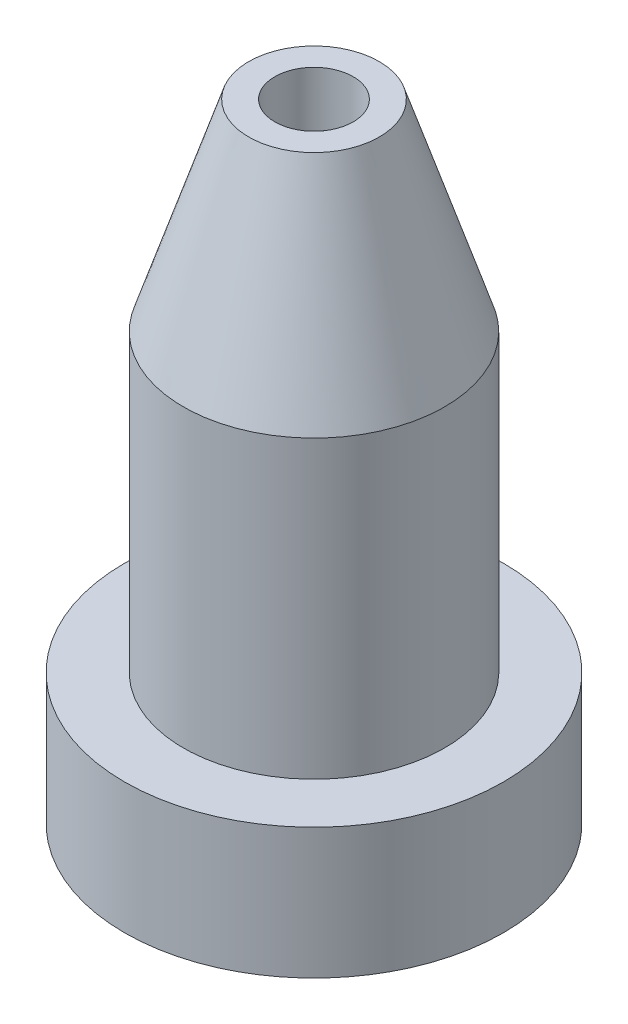
from build123d import *

# Parameters (mm, degrees)
SKETCH1_R           = 1
BOSS_EXTRUDE1_DEPTH = 4.8
SKETCH3_R           = 0.75
CUT_EXTRUDE1_DEPTH  = 3
SKETCH4_R           = 0.3
CUT_EXTRUDE2_DEPTH  = 3
SKETCH5_R           = 0.5
CUT_EXTRUDE3_DEPTH  = 0.6
SKETCH6_R           = 1.45
SKETCH6_R_2         = 1
BOSS_EXTRUDE2_DEPTH = 1
CHAMFER1_SIZE       = 0.3
CHAMFER1_SIZE2      = 1


with BuildPart() as part:
    # Sketch1 → Boss-Extrude1 (new body)
    with BuildSketch(Plane(origin=(0, 0, 0), x_dir=(1, 0, 0), z_dir=(0, 1, 0))):
        with Locations(Location((0, 0, 0), (0, 0, 270))):
            Circle(SKETCH1_R)
    extrude(amount=BOSS_EXTRUDE1_DEPTH)

    # Sketch2 → Cut-Revolve1 (revolve, cut)
    with BuildSketch(Plane.XY, mode=Mode.PRIVATE) as cut_revolve1_sk:
        Polygon((0.5, 4.8), (1.621441373, 1.348558349), (1.621441373, 4.8), align=None)
    revolve(cut_revolve1_sk.sketch.rotate(Axis((0, 0, 0), (0, 1, 0)), 90), axis=Axis((0, 0, 0), (0, 1, 0)), mode=Mode.SUBTRACT)

    # Sketch3 → Cut-Extrude1 (cut)
    with BuildSketch(Plane.XZ):
        with Locations(Location((0, 0, 0), (0, 0, 270))):
            Circle(SKETCH3_R)
    extrude(amount=-CUT_EXTRUDE1_DEPTH, mode=Mode.SUBTRACT)

    # Sketch4 → Cut-Extrude2 (cut)
    with BuildSketch(Plane(origin=(0, 4.8, 0), x_dir=(1, 0, 0), z_dir=(0, 1, 0))):
        with Locations(Location((0, 0, 0), (0, 0, 270))):
            Circle(SKETCH4_R)
    extrude(amount=-CUT_EXTRUDE2_DEPTH, mode=Mode.SUBTRACT)

    # Sketch5 → Cut-Extrude3 (cut)
    with BuildSketch(Plane.XZ.offset(-3)):
        with Locations(Location((0, 0, 0), (0, 0, 270))):
            Circle(SKETCH5_R)
    extrude(amount=-CUT_EXTRUDE3_DEPTH, mode=Mode.SUBTRACT)

    # Sketch6 → Boss-Extrude2 (add)
    with BuildSketch(Plane.XZ):
        with Locations(Location((0, 0, 0), (0, 0, 270))):
            Circle(SKETCH6_R)
        with Locations(Location((0, 0, 0), (0, 0, 270))):
            Circle(SKETCH6_R_2, mode=Mode.SUBTRACT)
    extrude(amount=-BOSS_EXTRUDE2_DEPTH)

    # Chamfer1
    chamfer1_edges = [part.edges().sort_by_distance(p)[0] for p in [
        (0, 0, 0.75),
    ]]
    chamfer1_side = [part.faces().sort_by_distance(p)[0] for p in [
        (0, 0, 1.408987807),
    ]]
    chamfer(chamfer1_edges, length=CHAMFER1_SIZE, length2=CHAMFER1_SIZE2, reference=chamfer1_side[0])


solid = part.part
